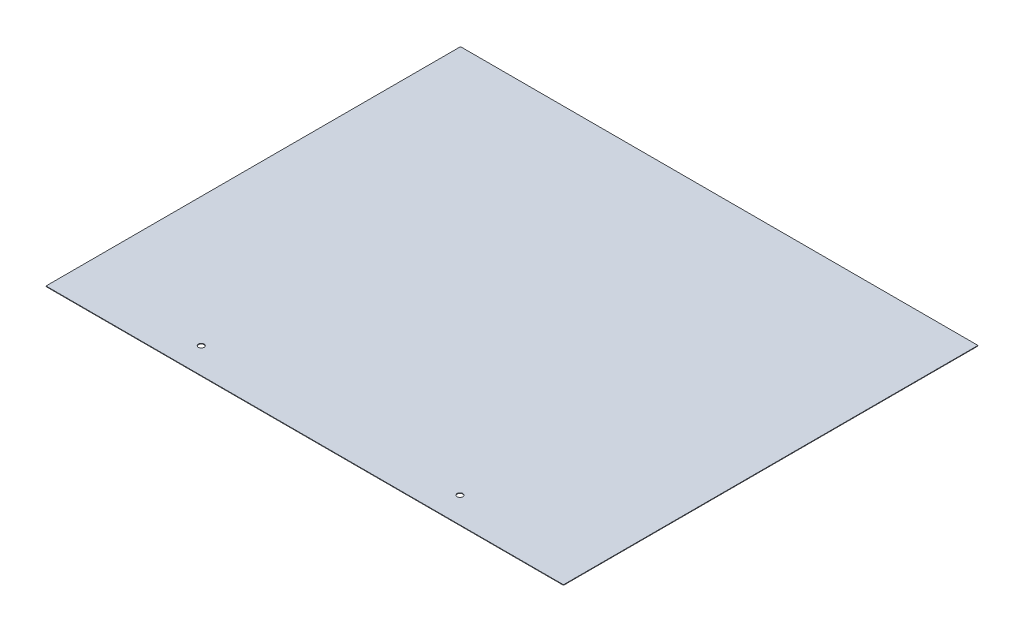
from build123d import *

# Parameters (mm, degrees)
SKETCH1_W           = 1000
SKETCH1_H           = 801
BOSS_EXTRUDE1_DEPTH = 1
SKETCH2_R           = 5.5
CUT_EXTRUDE1_DEPTH  = 641.625670731


with BuildPart() as part:
    # Sketch1 → Boss-Extrude1 (new body)
    with BuildSketch(Plane(origin=(0, 0, 0), x_dir=(1, 0, 0), z_dir=(0, 1, 0))):
        Rectangle(SKETCH1_W, SKETCH1_H)
    extrude(amount=BOSS_EXTRUDE1_DEPTH)

    # Sketch2 → Cut-Extrude1 (cut, through all)
    with BuildSketch(Plane(origin=(0, 1, 0), x_dir=(1, 0, 0), z_dir=(0, 1, 0))):
        with Locations(Location((-250, -350.5, 0), (0, 0, 270))):
            Circle(SKETCH2_R)
        with Locations(Location((250, -350.5, 0), (0, 0, 270))):
            Circle(SKETCH2_R)
    extrude(amount=-CUT_EXTRUDE1_DEPTH, mode=Mode.SUBTRACT)


solid = part.part
